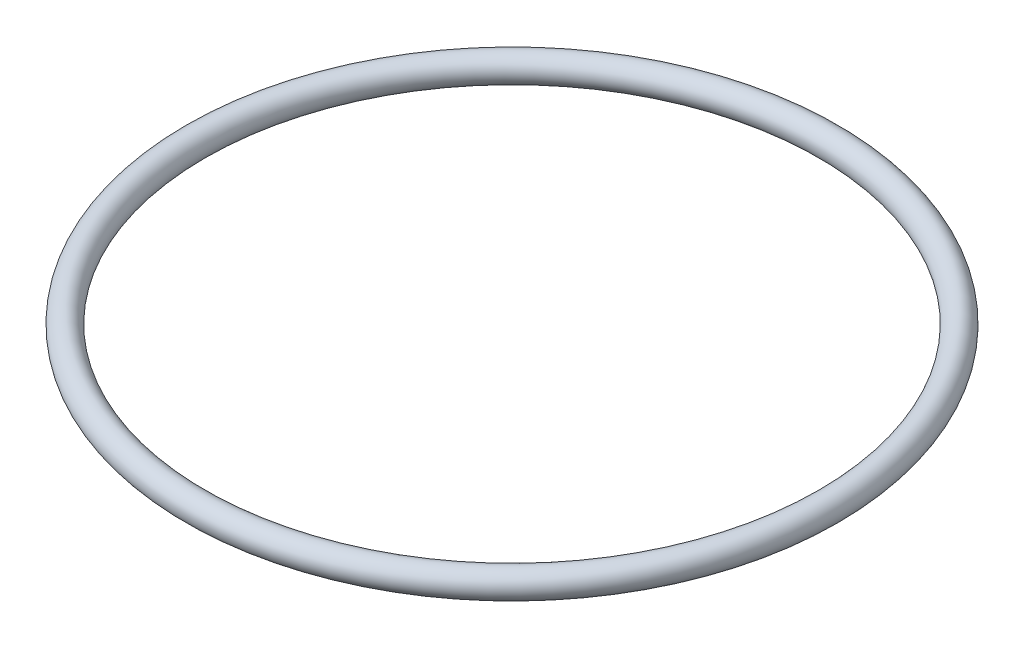
from build123d import *

# Parameters (mm, degrees)
SKETCH1_R = 1.5


with BuildPart() as part:
    # Sketch1 → Revolve1 (revolve)
    with BuildSketch(Plane.XY):
        with Locations((-86.031169153, -104.0167177)):
            Circle(SKETCH1_R)
    revolve(axis=Axis((-121.531169153, -142.3167177, 0), (0, 1, 0)))


solid = part.part
